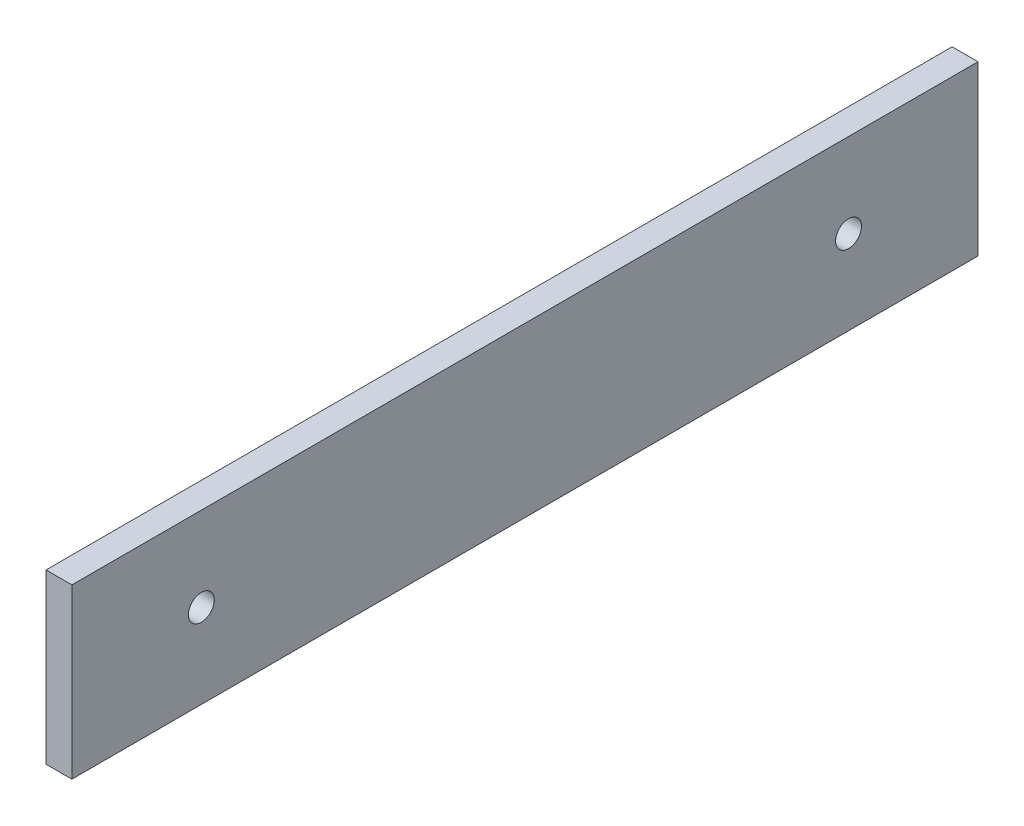
from build123d import *

# Parameters (mm, degrees)
SKETCH1_W           = 700
SKETCH1_H           = 130
SKETCH1_R           = 10
BOSS_EXTRUDE1_DEPTH = 20


with BuildPart() as part:
    # Sketch1 → Boss-Extrude1 (new body)
    with BuildSketch(Plane(origin=(0, 0, 0), x_dir=(0, 0, -1), z_dir=(1, 0, 0))):
        Rectangle(SKETCH1_W, SKETCH1_H)
        with Locations((-250, 0)):
            Circle(SKETCH1_R, mode=Mode.SUBTRACT)
        with Locations((250, 0)):
            Circle(SKETCH1_R, mode=Mode.SUBTRACT)
    extrude(amount=BOSS_EXTRUDE1_DEPTH)


solid = part.part
